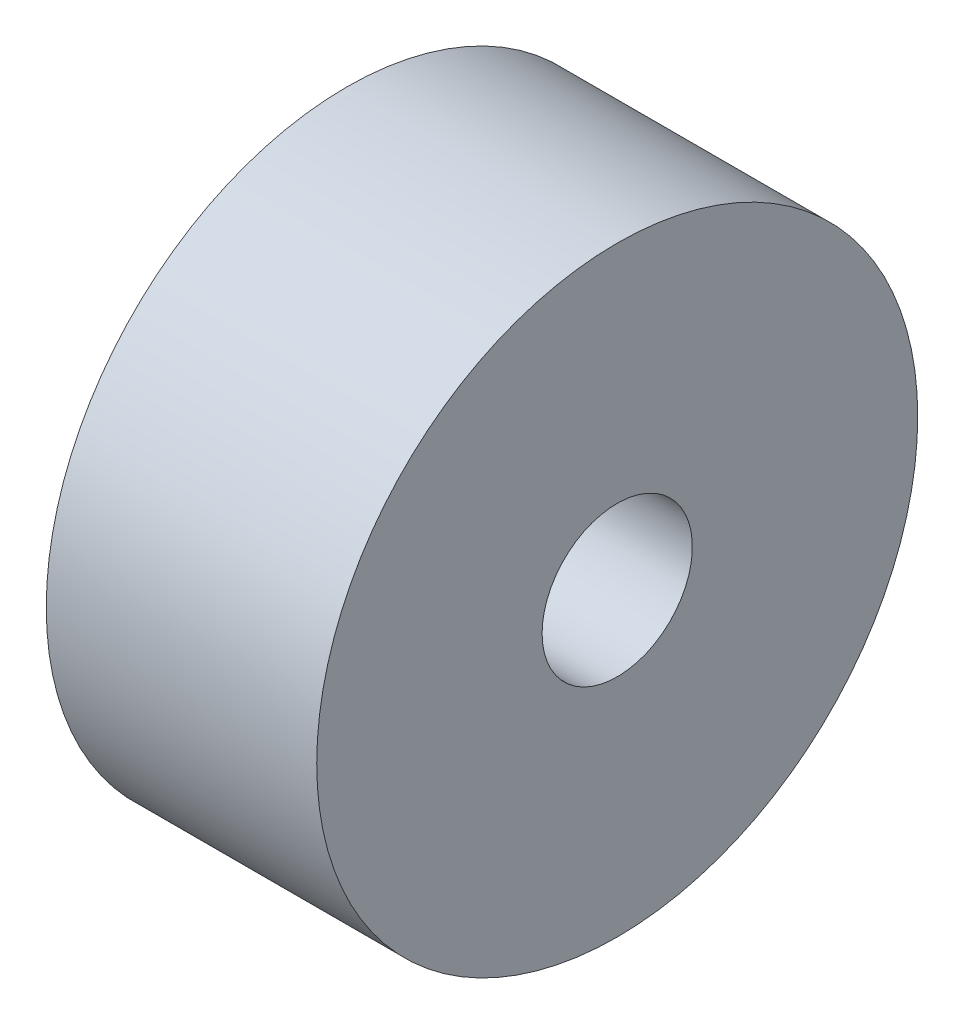
from build123d import *

# Parameters (mm, degrees)
SKETCH1_W = 36
SKETCH1_H = 30


with BuildPart() as part:
    # Sketch1 → Revolve1 (revolve)
    with BuildSketch(Plane.XY, mode=Mode.PRIVATE) as revolve1_sk:
        with Locations((0, 25)):
            Rectangle(SKETCH1_W, SKETCH1_H)
    revolve(revolve1_sk.sketch.rotate(Axis((-109.713732369, 0, 0), (1, 0, 0)), 90), axis=Axis((-109.713732369, 0, 0), (1, 0, 0)))


solid = part.part
